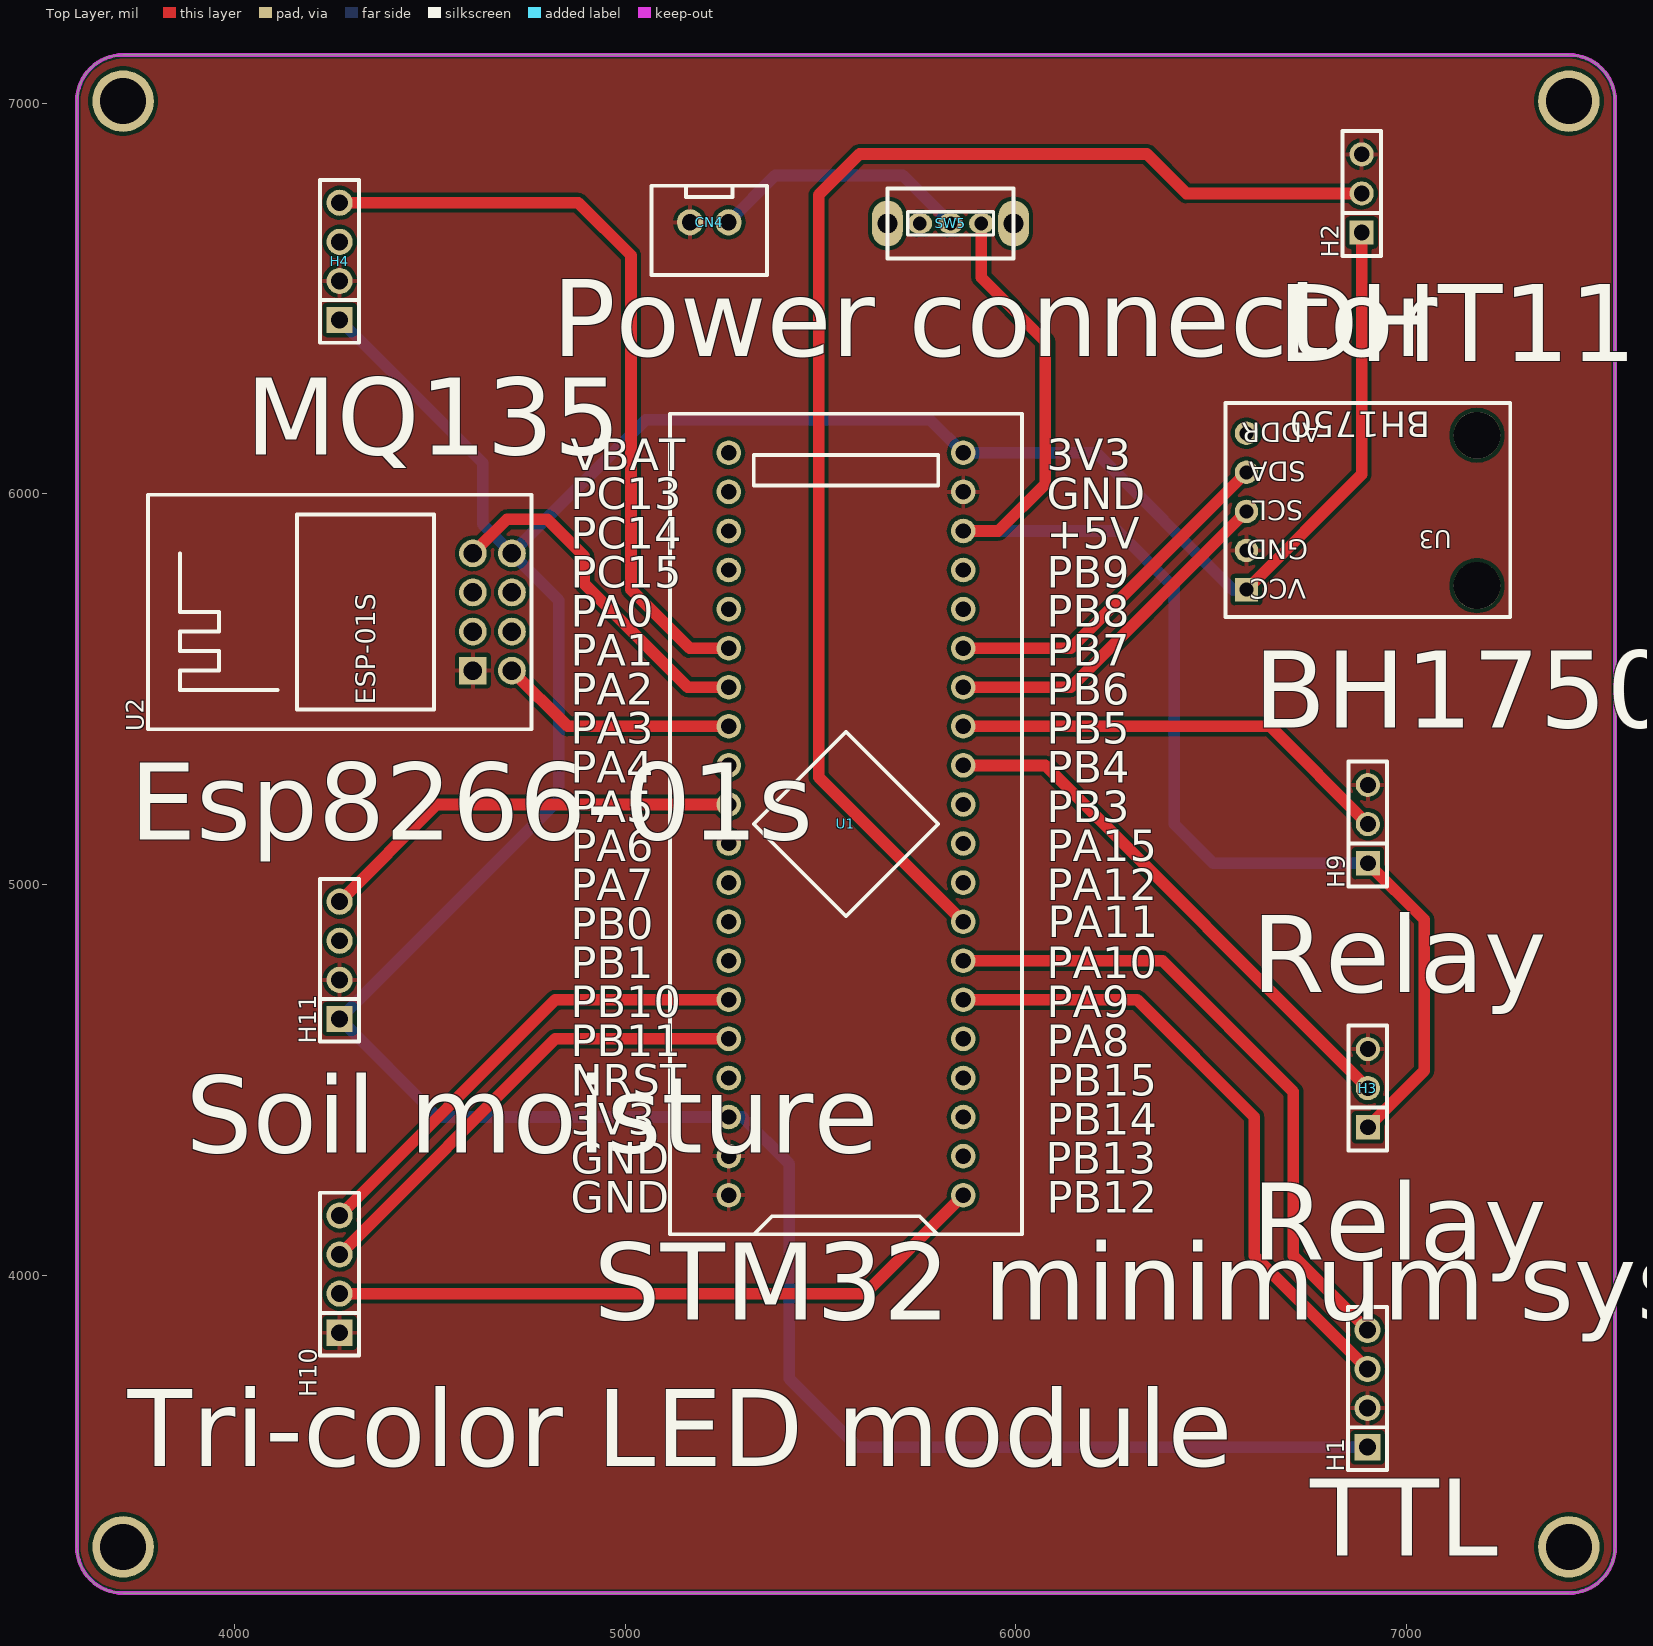
[diagram p0: Top Layer view]
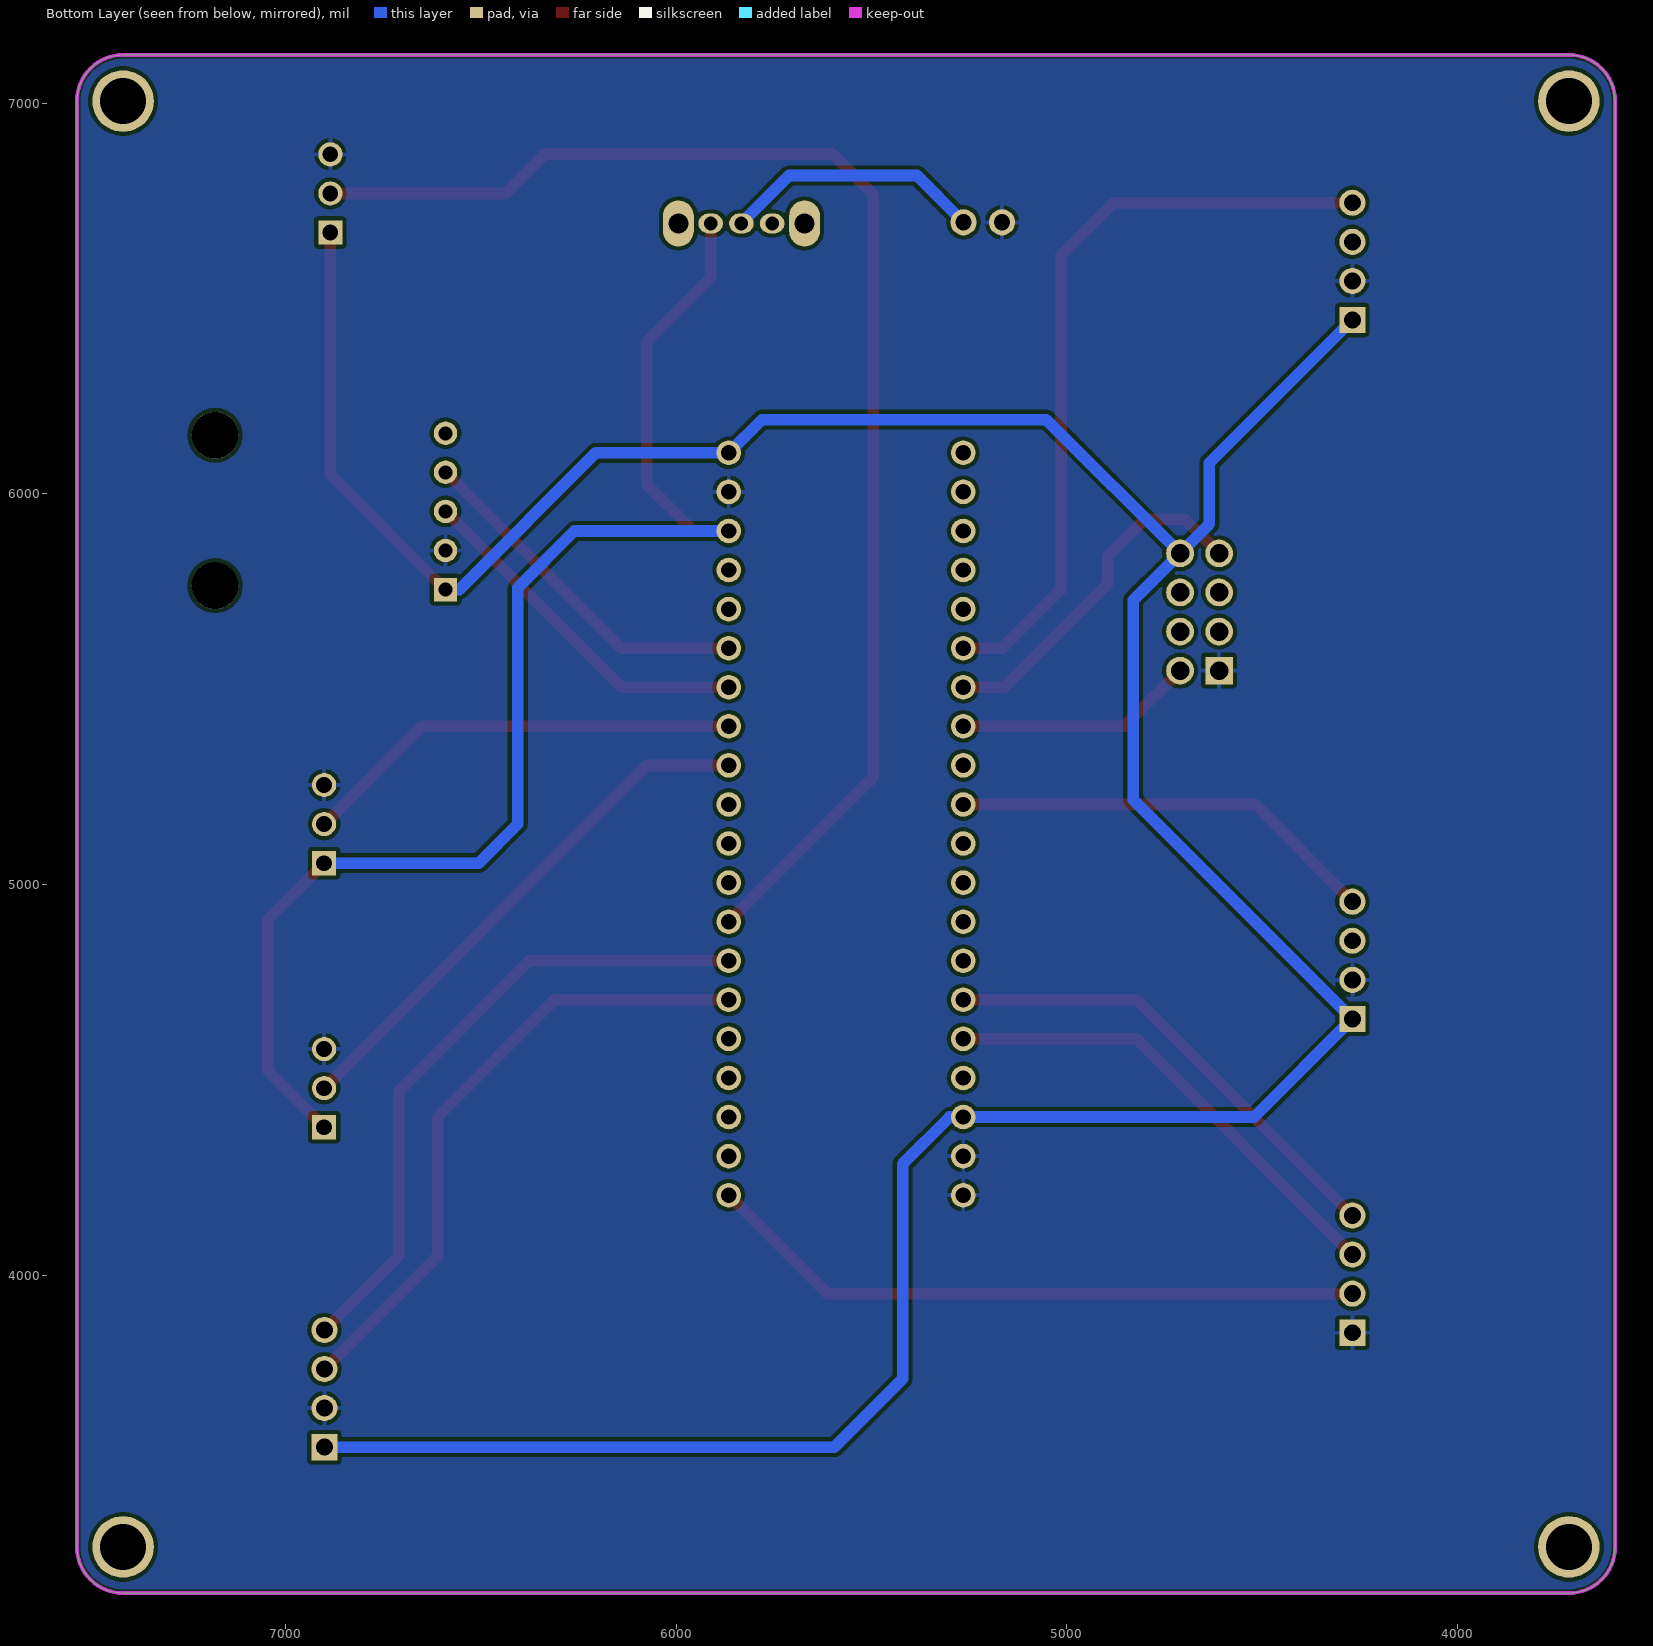
[diagram p1: Bottom Layer view, seen from below]
# Altium PCB MISC79011.pcbdoc
Units mil, origin at the board's own origin, x right, y up, seen from the top; angles counter-clockwise.
Board outline 3937.01 x 3937.01 mil, 2 copper layers (Top Layer, Bottom Layer), stack 62.206 mil thick; 12 components, 38 nets, 91 pads, 0 vias.

## Layer stack, top to bottom
Top Solder Mask Layer: solder mask 0.394, Dk 3.3
Top Layer: signal copper 1.379
Dielectric1: surface 59.449, FR4, Dk 4.5
Bottom Layer: signal copper 1.378
Bottom Solder Mask Layer: solder mask 0.394, Dk 3.3

## Board outline
3714.61,7123.5 ccw(c3714.61,7005.39) 3596.5,7005.39 3596.5,3304.61 ccw(c3714.61,3304.61) 3714.61,3186.5 7415.39,3186.5 ccw(c7415.39,3304.61) 7533.5,3304.61 7533.5,7005.39 ccw(c7415.39,7005.39) 7415.39,7123.5 3714.61,7123.5

## Design rules (kind name [scope] priority, off if disabled: settings)
BoardOutlineClearance copperThickness2oz_1 [All] p2 off: genericclearance=7.99 ignorepadtopadclearanceinfootprint=FALSE except(0: Arc-SplitContinuation Track-SplitContinuation SMDPad-SplitContinuation THPad-SplitContinuation Via-SplitContinuation Fill-SplitContinuation Region-SplitContinuation Poly-SplitContinuation Text-SplitContinuation Hole-SplitContinuation; 5.98: Arc-CutoutEdge Track-CutoutEdge SMDPad-CutoutEdge THPad-CutoutEdge Via-CutoutEdge Text-CutoutEdge; 6.9: Hole-OutlineEdge Hole-CutoutEdge; 10: Poly-OutlineEdge Poly-CutoutEdge; 11.81: Arc-OutlineEdge Track-OutlineEdge SMDPad-OutlineEdge THPad-OutlineEdge Via-OutlineEdge Fill-OutlineEdge Region-OutlineEdge Text-OutlineEdge Fill-CutoutEdge Region-CutoutEdge)
BoardOutlineClearance Plane_innerPlane_1 [All] p4 off: genericclearance=4.02 ignorepadtopadclearanceinfootprint=FALSE except(0: Arc-SplitContinuation Track-SplitContinuation SMDPad-SplitContinuation THPad-SplitContinuation Via-SplitContinuation Fill-SplitContinuation Region-SplitContinuation Poly-SplitContinuation Text-SplitContinuation Hole-SplitContinuation; 5.98: Arc-CutoutEdge Track-CutoutEdge SMDPad-CutoutEdge THPad-CutoutEdge Via-CutoutEdge Text-CutoutEdge; 6.9: Hole-OutlineEdge Hole-CutoutEdge; 10: Poly-OutlineEdge Poly-CutoutEdge; 11.81: Arc-OutlineEdge Track-OutlineEdge SMDPad-OutlineEdge THPad-OutlineEdge Via-OutlineEdge Fill-OutlineEdge Region-OutlineEdge Text-OutlineEdge Fill-CutoutEdge Region-CutoutEdge)
BoardOutlineClearance Copper_copperRegion_1 [All] p6 off: genericclearance=4.02 ignorepadtopadclearanceinfootprint=FALSE except(0: Arc-SplitContinuation Track-SplitContinuation SMDPad-SplitContinuation THPad-SplitContinuation Via-SplitContinuation Fill-SplitContinuation Region-SplitContinuation Poly-SplitContinuation Text-SplitContinuation Hole-SplitContinuation; 5.98: Arc-CutoutEdge Track-CutoutEdge SMDPad-CutoutEdge THPad-CutoutEdge Via-CutoutEdge Text-CutoutEdge; 6.9: Hole-OutlineEdge Hole-CutoutEdge; 10: Poly-OutlineEdge Poly-CutoutEdge; 11.81: Arc-OutlineEdge Track-OutlineEdge SMDPad-OutlineEdge THPad-OutlineEdge Via-OutlineEdge Fill-OutlineEdge Region-OutlineEdge Text-OutlineEdge Fill-CutoutEdge Region-CutoutEdge)
BoardOutlineClearance Copper_copperRegion_copperThickness1oz_1 [All] p8 off: genericclearance=4.02 ignorepadtopadclearanceinfootprint=FALSE except(0: Arc-SplitContinuation Track-SplitContinuation SMDPad-SplitContinuation THPad-SplitContinuation Via-SplitContinuation Fill-SplitContinuation Region-SplitContinuation Poly-SplitContinuation Text-SplitContinuation Hole-SplitContinuation; 5.98: Arc-CutoutEdge Track-CutoutEdge SMDPad-CutoutEdge THPad-CutoutEdge Via-CutoutEdge Text-CutoutEdge; 6.9: Hole-OutlineEdge Hole-CutoutEdge; 10: Poly-OutlineEdge Poly-CutoutEdge; 11.81: Arc-OutlineEdge Track-OutlineEdge SMDPad-OutlineEdge THPad-OutlineEdge Via-OutlineEdge Fill-OutlineEdge Region-OutlineEdge Text-OutlineEdge Fill-CutoutEdge Region-CutoutEdge)
BoardOutlineClearance Copper_copperRegion_Copper_copperRegion_1 [All] p10 off: genericclearance=4.02 ignorepadtopadclearanceinfootprint=FALSE except(0: Arc-SplitContinuation Track-SplitContinuation SMDPad-SplitContinuation THPad-SplitContinuation Via-SplitContinuation Fill-SplitContinuation Region-SplitContinuation Poly-SplitContinuation Text-SplitContinuation Hole-SplitContinuation; 5.98: Arc-CutoutEdge Track-CutoutEdge SMDPad-CutoutEdge THPad-CutoutEdge Via-CutoutEdge Text-CutoutEdge; 6.9: Hole-OutlineEdge Hole-CutoutEdge; 10: Poly-OutlineEdge Poly-CutoutEdge; 11.81: Arc-OutlineEdge Track-OutlineEdge SMDPad-OutlineEdge THPad-OutlineEdge Via-OutlineEdge Fill-OutlineEdge Region-OutlineEdge Text-OutlineEdge Fill-CutoutEdge Region-CutoutEdge)
BoardOutlineClearance copperThickness1oz_1 [All] p12: genericclearance=4.02 ignorepadtopadclearanceinfootprint=FALSE except(0: Arc-SplitContinuation Track-SplitContinuation SMDPad-SplitContinuation THPad-SplitContinuation Via-SplitContinuation Fill-SplitContinuation Region-SplitContinuation Poly-SplitContinuation Text-SplitContinuation Hole-SplitContinuation; 5.98: Arc-CutoutEdge Track-CutoutEdge SMDPad-CutoutEdge THPad-CutoutEdge Via-CutoutEdge Text-CutoutEdge; 6.9: Hole-OutlineEdge Hole-CutoutEdge; 10: Poly-OutlineEdge Poly-CutoutEdge; 11.81: Arc-OutlineEdge Track-OutlineEdge SMDPad-OutlineEdge THPad-OutlineEdge Via-OutlineEdge Fill-OutlineEdge Region-OutlineEdge Text-OutlineEdge Fill-CutoutEdge Region-CutoutEdge)
Clearance copperThickness2oz [All] p1 off: gap=7.99 ignorepadtopadclearanceinfootprint=FALSE except(5.98: SMDPad-Track SMDPad-SMDPad THPad-Track SMDPad-THPad THPad-THPad Track-Via SMDPad-Via THPad-Via Via-Via Fill-SMDPad Region-SMDPad Fill-THPad Region-THPad Fill-Via Region-Via Fill-Fill Fill-Region Region-Region Arc-Track Arc-SMDPad Arc-THPad Arc-Via Fill-Arc Region-Arc Arc-Arc Text-Track SMDPad-Text Text-THPad Text-Via Fill-Text Region-Text Arc-Text Text-Text; 6.9: Hole-Track Hole-SMDPad Hole-THPad Hole-Via Fill-Hole Region-Hole Hole-Arc Hole-Text; 10: Poly-Track Poly-SMDPad Poly-THPad Poly-Via Poly-Fill Poly-Region Poly-Poly Poly-Arc Poly-Text Poly-Hole; 11.81: Fill-Track Region-Track)
Clearance Plane_innerPlane [All] p3 off: gap=4.02 ignorepadtopadclearanceinfootprint=FALSE except(5.98: SMDPad-Track SMDPad-SMDPad THPad-Track SMDPad-THPad THPad-THPad Track-Via SMDPad-Via THPad-Via Via-Via Fill-SMDPad Region-SMDPad Fill-THPad Region-THPad Fill-Via Region-Via Fill-Fill Fill-Region Region-Region Arc-Track Arc-SMDPad Arc-THPad Arc-Via Fill-Arc Region-Arc Arc-Arc Text-Track SMDPad-Text Text-THPad Text-Via Fill-Text Region-Text Arc-Text Text-Text; 6.9: Hole-Track Hole-SMDPad Hole-THPad Hole-Via Fill-Hole Region-Hole Hole-Arc Hole-Text; 10: Poly-Track Poly-SMDPad Poly-THPad Poly-Via Poly-Fill Poly-Region Poly-Poly Poly-Arc Poly-Text Poly-Hole; 11.81: Fill-Track Region-Track)
Clearance Copper_copperRegion [All] p5 off: gap=4.02 ignorepadtopadclearanceinfootprint=FALSE except(5.98: SMDPad-Track SMDPad-SMDPad THPad-Track SMDPad-THPad THPad-THPad Track-Via SMDPad-Via THPad-Via Via-Via Fill-SMDPad Region-SMDPad Fill-THPad Region-THPad Fill-Via Region-Via Fill-Fill Fill-Region Region-Region Arc-Track Arc-SMDPad Arc-THPad Arc-Via Fill-Arc Region-Arc Arc-Arc Text-Track SMDPad-Text Text-THPad Text-Via Fill-Text Region-Text Arc-Text Text-Text; 6.9: Hole-Track Hole-SMDPad Hole-THPad Hole-Via Fill-Hole Region-Hole Hole-Arc Hole-Text; 10: Poly-Track Poly-SMDPad Poly-THPad Poly-Via Poly-Fill Poly-Region Poly-Poly Poly-Arc Poly-Text Poly-Hole; 11.81: Fill-Track Region-Track)
Clearance Copper_copperRegion_copperThickness1oz [All] p7 off: gap=4.02 ignorepadtopadclearanceinfootprint=FALSE except(5.98: SMDPad-Track SMDPad-SMDPad THPad-Track SMDPad-THPad THPad-THPad Track-Via SMDPad-Via THPad-Via Via-Via Fill-SMDPad Region-SMDPad Fill-THPad Region-THPad Fill-Via Region-Via Fill-Fill Fill-Region Region-Region Arc-Track Arc-SMDPad Arc-THPad Arc-Via Fill-Arc Region-Arc Arc-Arc Text-Track SMDPad-Text Text-THPad Text-Via Fill-Text Region-Text Arc-Text Text-Text; 6.9: Hole-Track Hole-SMDPad Hole-THPad Hole-Via Fill-Hole Region-Hole Hole-Arc Hole-Text; 10: Poly-Track Poly-SMDPad Poly-THPad Poly-Via Poly-Fill Poly-Region Poly-Poly Poly-Arc Poly-Text Poly-Hole; 11.81: Fill-Track Region-Track)
Clearance Copper_copperRegion_Copper_copperRegion [All] p9 off: gap=4.02 ignorepadtopadclearanceinfootprint=FALSE except(5.98: SMDPad-Track SMDPad-SMDPad THPad-Track SMDPad-THPad THPad-THPad Track-Via SMDPad-Via THPad-Via Via-Via Fill-SMDPad Region-SMDPad Fill-THPad Region-THPad Fill-Via Region-Via Fill-Fill Fill-Region Region-Region Arc-Track Arc-SMDPad Arc-THPad Arc-Via Fill-Arc Region-Arc Arc-Arc Text-Track SMDPad-Text Text-THPad Text-Via Fill-Text Region-Text Arc-Text Text-Text; 6.9: Hole-Track Hole-SMDPad Hole-THPad Hole-Via Fill-Hole Region-Hole Hole-Arc Hole-Text; 10: Poly-Track Poly-SMDPad Poly-THPad Poly-Via Poly-Fill Poly-Region Poly-Poly Poly-Arc Poly-Text Poly-Hole; 11.81: Fill-Track Region-Track)
Clearance copperThickness1oz [All] p11: gap=4.02 ignorepadtopadclearanceinfootprint=FALSE except(5.98: SMDPad-Track SMDPad-SMDPad THPad-Track SMDPad-THPad THPad-THPad Track-Via SMDPad-Via THPad-Via Via-Via Fill-SMDPad Region-SMDPad Fill-THPad Region-THPad Fill-Via Region-Via Fill-Fill Fill-Region Region-Region Arc-Track Arc-SMDPad Arc-THPad Arc-Via Fill-Arc Region-Arc Arc-Arc Text-Track SMDPad-Text Text-THPad Text-Via Fill-Text Region-Text Arc-Text Text-Text; 6.9: Hole-Track Hole-SMDPad Hole-THPad Hole-Via Fill-Hole Region-Hole Hole-Arc Hole-Text; 10: Poly-Track Poly-SMDPad Poly-THPad Poly-Via Poly-Fill Poly-Region Poly-Poly Poly-Arc Poly-Text Poly-Hole; 11.81: Fill-Track Region-Track)
DiffPairsRouting differentialPair [All] p1: maxlimit=6 minlimit=6 mostfreqgap=6 toplayer_minwidth=5 toplayer_prefwidth=10 toplayer_maxwidth=100 toplayer_mingap=6 toplayer_prefgap=6 toplayer_maxgap=6 bottomlayer_minwidth=5 bottomlayer_prefwidth=10 bottomlayer_maxwidth=100 bottomlayer_mingap=6 bottomlayer_prefgap=6 bottomlayer_maxgap=6 maxuncoupledlength=10
HoleToHoleClearance otherClearance [All] p1: gap=11.81 allowstackedmicrovias=TRUE
Length netLength [All] p1: minlimit=0 maxlimit=0
PasteMaskExpansion pasteMaskExpansion [All] p1: expansion=0
PlaneConnect innerPlane [All] p1: planeconnectstyle=Relief reliefexpansion=20 reliefentries=4 reliefconductorwidth=10 reliefairgap=10
PolygonConnect copperRegion_copperThickness1oz [All] p1 off: connectstyle=Relief reliefconductorwidth=10 reliefentries=4 polygonreliefangle="90 Angle" airgapwidth=10 via.connectstyle=Relief via.reliefconductorwidth=10 via.reliefentries=4 via.polygonreliefangle="90 Angle" via.airgapwidth=10
PolygonConnect copperRegion_Copper_copperRegion [All] p2 off: connectstyle=Relief reliefconductorwidth=10 reliefentries=4 polygonreliefangle="90 Angle" airgapwidth=10 via.connectstyle=Relief via.reliefconductorwidth=10 via.reliefentries=4 via.polygonreliefangle="90 Angle" via.airgapwidth=10
PolygonConnect copperRegion [All] p3: connectstyle=Relief reliefconductorwidth=10 reliefentries=4 polygonreliefangle="90 Angle" airgapwidth=10 via.connectstyle=Relief via.reliefconductorwidth=10 via.reliefentries=4 via.polygonreliefangle="90 Angle" via.airgapwidth=10
RoutingVias viaSize [All] p1: holewidth=12.01 width=24.02 viastyle="Through Hole" minholewidth=11.81 minwidth=19.68 maxholewidth=248.03 maxwidth=393.7
SolderMaskExpansion solderMaskExpansion [IsVia] p1: expansion=-1000 istentingtop=TRUE
SolderMaskExpansion solderMaskExpansion [All] p2: expansion=2 istentingtop=FALSE
Width copperThickness2oz_2 [All] p1 off: maxlimit=100 minlimit=8 preferedwidth=10
Width copperThickness1oz_2 [All] p2: maxlimit=100 minlimit=5 preferedwidth=10

## Components (designator, comment, footprint, x,y, rotation, side; value= is the part's Value field where it differs from the comment)
CN4 "XH2.54*2P_straight" CONN-TH_2P-P2.50-XH2.54-2P 5215,6695 r0 top
H1 "" HDR-TH_4P-P2.54-V-F 6900,3710 r90 top
H2 "" HDR-TH_3P-P2.54-V-F 6884.74,6768.84 r90 top
H3 "" HDR-TH_3P-P2.54-V-F 6900.83,4478.99 r90 top
H4 "" HDR-TH_4P-P2.54-V-F 4269,6595 r90 top
H9 "" HDR-TH_3P-P2.54-V-F 6900.83,5154.76 r90 top
H10 "" HDR-TH_4P-P2.54-V-F 4269,4002.95 r90 top
H11 "" HDR-TH_4P-P2.54-V-F 4269,4806.14 r90 top
SW5 "" 拨动开关 5837.9,6692.05 r180 top
U1 "STM32F103C8T6-Card" CONN-TH_L53.3-W22.9_STM32F103C8T6-CARD 5565,5155 r90 top
U2 "ESP-01S" WIFIM-TH_ESP-01S 4660,5697.59 r90 top
U3 "" BH1750光照传感器 6850,5965 r180 top

## Footprints (in the part's own frame and the unit in brackets; to place one, negate y for a bottom-side part, rotate by r counter-clockwise, add the part's x,y. Pads: shape width x height; smd on the part's side, far side on the other; paste and mask are expansions set on the pad)
BH1750光照传感器 [mil]
  rect 60x60 hole 36: 1(260,210)
  round 60 hole 36: 2(260,110) 3(260,10) 4(260,-90) 5(260,-190)
  round 120 hole 120 unplated: ""(-330,-185) ""(-330,200)
  silkscreen extent -415,-267 313,280
CONN-TH_2P-P2.50-XH2.54-2P [mm]
  round 1.7 hole 1.05 paste+0 mask+0.05: 1(1.25,0) 2(-1.25,0)
  silkscreen extent -3.75,-3.42 3.75,2.37
CONN-TH_L53.3-W22.9_STM32F103C8T6-CARD [mm]
  round 1.6 hole 1: 1(-24.13,-7.62) 2(-21.59,-7.62) 3(-19.05,-7.62) 4(-16.51,-7.62) 5(-13.97,-7.62) 6(-11.43,-7.62) 7(-8.89,-7.62) 8(-6.35,-7.62) 9(-3.81,-7.62) 10(-1.27,-7.62) 11(1.27,-7.62) 12(3.81,-7.62) 13(6.35,-7.62) 14(8.89,-7.62) 15(11.43,-7.62) 16(13.97,-7.62) 17(16.51,-7.62) 18(19.05,-7.62) 19(21.59,-7.62) 20(24.13,-7.62) 21(24.13,7.62) 22(21.59,7.62) 23(19.05,7.62) 24(16.51,7.62) 25(13.97,7.62) 26(11.43,7.62) 27(8.89,7.62) 28(6.35,7.62) 29(3.81,7.62) 30(1.27,7.62) 31(-1.27,7.62) 32(-3.81,7.62) 33(-6.35,7.62) 34(-8.89,7.62) 35(-11.43,7.62) 36(-13.97,7.62) 37(-16.51,7.62) 38(-19.05,7.62) 39(-21.59,7.62) 40(-24.13,7.62)
  silkscreen extent -26.67,-11.43 26.67,11.43
HDR-TH_3P-P2.54-V-F [mil]
  rect 62x62 hole 40.16: 1(-100,0)
  round 62 hole 40.16: 2(0,0) 3(100,0)
  silkscreen extent -160,-49 160,49
HDR-TH_4P-P2.54-V-F [mm]
  rect 1.7x1.7 hole 1.1: 1(-3.81,0)
  round 1.7 hole 1.1: 2(-1.27,0) 3(1.27,0) 4(3.81,0)
  silkscreen extent -5.29,-1.27 5.29,1.27
WIFIM-TH_ESP-01S [mm]
  rect 1.8x1.8 hole 1.2: 1(-3.81,1.27)
  round 1.8 hole 1.2: 2(-1.27,1.27) 3(1.27,1.27) 4(3.81,1.27) 5(3.81,-1.27) 6(1.27,-1.27) 7(-1.27,-1.27) 8(-3.81,-1.27)
  silkscreen extent -7.62,-2.54 7.62,22.4
拨动开关 [mil]
  oval 63x51.2 hole 35.4 paste+0 mask+2: 1(-73.4,0) 2(5,0) 3(84,0)
  oval 78.7x118.1 hole 51.2 paste+0 mask+2: 4(166.7,0) 5(-156.1,0)
  silkscreen extent -156,-90 167,90

## Free pads (board coordinates)
  round 157.48 hole 118.11: 1(3714.61,7005.39) 1(3714.61,3304.61) 1(7415.39,7005.39) 1(7415.39,3304.61)

## Nets (pads, with @x,y where several pads share a name; then routed paths per layer and width w, separated by ;. In a path a pad name is that pad's centre, name@x,y a point inside that pad or via, vN(x,y) a via of type N, cw(c..) or ccw(c..) an arc to the next point about the centre after c; other vN are vias at no path point)
$1N17118: CN4.1 SW5.2 | length 669.3
  Bottom Layer w30: CN4.1 5384.22,6815 5709.95,6815 SW5.2
+5V: H3.1 H9.1 SW5.1 U1.18 | length 3532.2
  Top Layer w30: U1.18 5955,5905 6075,6025 6075,6390 5911.3,6553.7 SW5.1 ; H3.1 7045,4523.17 7045,4910.59 H9.1
  Bottom Layer w30: U1.18 6260,5905 6405,5760 6405,5155 6505.24,5054.76 H9.1
GND: CN4.2 H1.2 H2.3 H3.3 H4.2 H9.3 H10.1 H11.2 U1.19 U1.39 U1.40 U2.1 U3.2
NRST: U1.37
PA0: U1.25
PA1: H4.4 U1.26 | length 1969
  Top Layer w30: H4.4 4880,6745 5015,6610 5015,5755 5165,5605 U1.26
PA2: U1.27 U2.4 | length 910.3
  Top Layer w30: U2.4 4697.41,5935 4800,5935 4895,5840 4895,5770 5160,5505 U1.27
PA3: U1.28 U2.8 | length 614.1
  Top Layer w30: U2.8 4852.59,5405 U1.28
PA4: U1.29
PA5: H11.4 U1.30 | length 1099.1
  Top Layer w30: H11.4 4517.86,5205 U1.30
PA6: U1.31
PA7: U1.32
PA8: U1.5
PA9: H1.3 U1.6 | length 1634.4
  Top Layer w30: U1.6 6310,4705 6610,4405 6610,4050 H1.3
PA10: H1.4 U1.7 | length 1672.5
  Top Layer w30: U1.7 6375,4805 6710,4470 6710,4050 H1.4
PA11: H2.2 U1.8 | length 3488.4
  Top Layer w30: U1.8 5495,5275 5495,6765 5600,6870 6335,6870 6436.16,6768.84 H2.2
PA12: U1.9
PA15: U1.10
PB0: U1.33
PB1: U1.34
PB3: U1.11
PB4: H3.2 U1.12 | length 1378
  Top Layer w30: U1.12 6074.82,5305 H3.2
PB5: H9.2 U1.13 | length 1139.5
  Top Layer w30: U1.13 6650.58,5405 H9.2
PB6: U1.14 U3.3 | length 911.4
  Top Layer w30: U1.14 6140,5505 U3.3
PB7: U1.15 U3.4 | length 911.4
  Top Layer w30: U1.15 6140,5605 U3.4
PB8: U1.16
PB9: U1.17
PB10: H10.4 U1.35 | length 1224.7
  Top Layer w30: H10.4 4821.05,4705 U1.35
PB11: H10.3 U1.36 | length 1224.7
  Top Layer w30: H10.3 4821.05,4605 U1.36
PB12: H10.2 U1.1 | length 1700.4
  Top Layer w30: H10.2 5612.94,3952.95 U1.1
PB13: U1.2
PB14: U1.3
PB15: U1.4
PC13: U1.22
PC14: U1.23
PC15: U1.24
VBAT: U1.21
VCC: H1.1 H2.1 H4.1 H11.1 U1.20 U1.38 U2.5 U3.1 | length 8898.8
  Top Layer w30: U3.1 6884.74,6049.74 H2.1
  Bottom Layer w30: H4.1 4635,6079 4635,5922.59 U2.5 ; U3.1 6555,5755 6205,6105 U1.20 5780,6190 5052.41,6190 U2.5 ; H1.1 5595,3560 5420,3735 5420,4285 5300,4405 U1.38 4520.14,4405 H11.1 4830,5217.14 4830,5727.59 U2.5
pads on no net: H4.3 H11.3 SW5.3 SW5.4 SW5.5 U2.2 U2.3 U2.6 U2.7 U3. U3.5

## Polygon pours and split planes (outlines as drawn)
GND on Bottom Layer (solid, remove dead copper, pour order 2): 3525,7245 3525,3080 7700,3080 7700,7245
GND on Top Layer (solid, remove dead copper, pour order 2): 3000,7415 3000,3000 7930,3000 7930,7415

## Keep-outs
Board Outline Layer:
  the board outline again, w10

## Silkscreen, mask and mechanical layers (free items; w line width, h text height)
Top Silkscreen Layer:
  text "Power connector" at 4812.87,6351.57 h196.85
  text "DHT11" at 6670,6340 h196.85
  text "MQ135" at 4028.31,6100.64 h196.85
  text "VBAT" at 4860.95,6060 h80
  text "3V3" at 6079.16,6060 h80
  text "PC13" at 4860.95,5960 h80
  text "GND" at 6079.16,5960 h80
  text "PC14" at 4860.95,5860 h80
  text "+5V" at 6079.16,5860 h80
  text "PC15" at 4860.95,5760 h80
  text "PB9" at 6079.16,5760 h80
  text "PA0" at 4860.95,5660 h80
  text "PB8" at 6079.16,5660 h80
  text "PA1" at 4860.95,5560 h80
  text "PB7" at 6079.16,5560 h80
  text "PA2" at 4860.95,5460 h80
  text "PB6" at 6079.16,5460 h80
  text "BH1750" at 6609.13,5401.38 h196.85
  text "PA3" at 4860.95,5360 h80
  text "PB5" at 6079.16,5360 h80
  text "PA4" at 4860.95,5260 h80
  text "PB4" at 6079.16,5260 h80
  text "PA5" at 4860.95,5160 h80
  text "PB3" at 6079.16,5160 h80
  text "Esp8266-01s" at 3732.14,5114.38 h196.85
  text "PA6" at 4860.95,5060 h80
  text "PA15" at 6079.16,5060 h80
  text "PA7" at 4860.95,4960 h80
  text "PA12" at 6079.16,4960 h80
  text "PA11" at 6080.95,4865 h80
  text "PB0" at 4860.95,4860 h80
  text "PB1" at 4860.95,4760 h80
  text "PA10" at 6079.16,4760 h80
  text "Relay" at 6603.61,4725.01 h196.85
  text "PB10" at 4860.95,4660 h80
  text "PA9" at 6079.16,4660 h80
  text "PB11" at 4860.95,4560 h80
  text "PA8" at 6079.16,4560 h80
  text "NRST" at 4860.95,4460 h80
  text "PB15" at 6079.16,4460 h80
  text "3V3" at 4860.95,4360 h80
  text "PB14" at 6079.16,4360 h80
  text "Soil moisture" at 3875.75,4312.98 h196.85
  text "GND" at 4860.95,4260 h80
  text "PB13" at 6075.95,4260 h80
  text "GND" at 4860.95,4160 h80
  text "PB12" at 6079.16,4160 h80
  text "Relay" at 6603.61,4040 h196.85
  text "STM32 minimum system" at 4919.45,3886.57 h196.85
  text "Tri-color LED module" at 3726.65,3511.57 h196.85
  text "TTL" at 6752.96,3281.57 h196.85